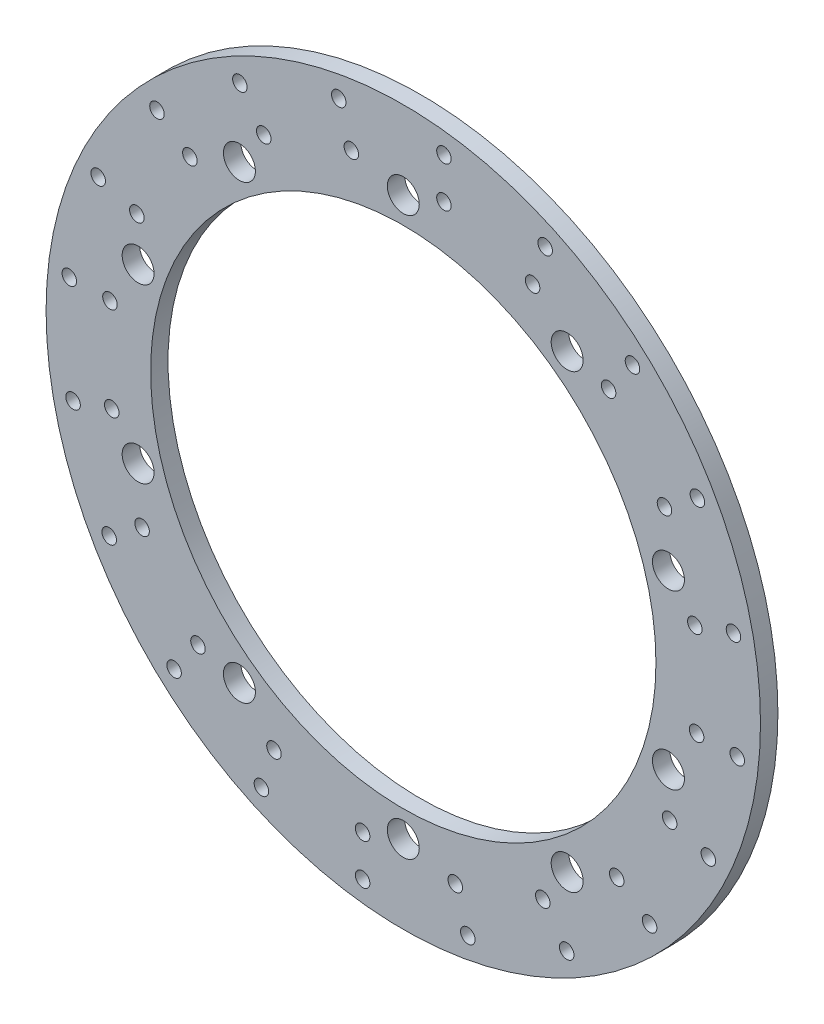
from build123d import *

# Parameters (mm, degrees)
SKETCH_1_R               = 61.5
SKETCH_1_R_2             = 43.5
EXTRUDE_1_DEPTH          = 1.5
HOLE_WIZARD_5_5_5_5_2_D  = 5.5
HOLE_WIZARD_M3_1_D       = 2.5
PATTERN_CIRCULAR_1_COUNT = 10
PATTERN_CIRCULAR_2_COUNT = 20


with BuildPart() as part:
    # 草图1 → 凸台-拉伸1 (new, symmetric)
    with BuildSketch(Plane.XY):
        Circle(SKETCH_1_R)
        Circle(SKETCH_1_R_2, mode=Mode.SUBTRACT)
    extrude(amount=EXTRUDE_1_DEPTH, both=True)

    # Ø5.5 (5.5) 直径孔2 (through all)
    with Locations(Plane.XY.offset(1.5)):
        with Locations((0, 48)):
            hole_wizard_5_5_5_5_2 = Hole(HOLE_WIZARD_5_5_5_5_2_D / 2)

    # M3 螺纹孔1 (through all)
    with Locations(Plane.XY.offset(1.5)):
        with Locations((-57.5, 7), (-50.5, 7)):
            hole_wizard_m3_1 = Hole(HOLE_WIZARD_M3_1_D / 2)

    # 阵列(圆周)1: Ø5.5 (5.5) 直径孔2 ×10 about axis
    pattern_circular_1_axis = Axis((0, 0, 0), (0, 0, 1))
    for i in range(1, PATTERN_CIRCULAR_1_COUNT):
        add(hole_wizard_5_5_5_5_2.rotate(pattern_circular_1_axis, i * 360 / PATTERN_CIRCULAR_1_COUNT), mode=Mode.SUBTRACT)

    # 阵列(圆周)2: M3 螺纹孔1 ×20 about axis
    pattern_circular_2_axis = Axis((0, 0, 0), (0, 0, 1))
    for i in range(1, PATTERN_CIRCULAR_2_COUNT):
        add(hole_wizard_m3_1.rotate(pattern_circular_2_axis, i * 360 / PATTERN_CIRCULAR_2_COUNT), mode=Mode.SUBTRACT)


solid = part.part
